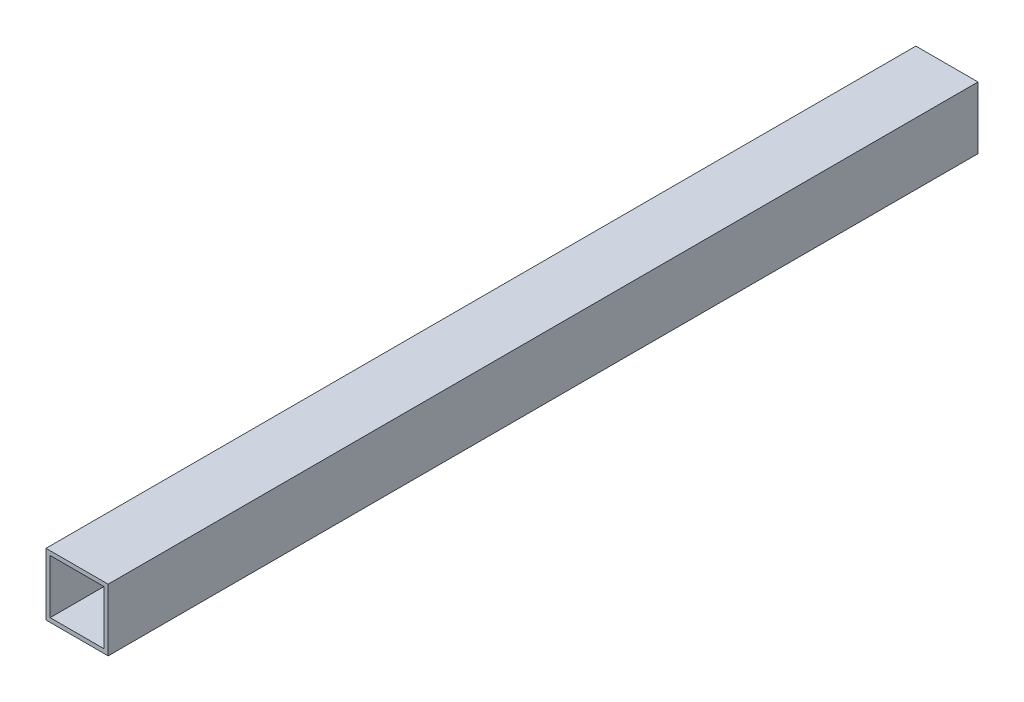
SolidWorks part; units mm, degrees
ref_plane "前视基准面" through (0, 0, 0) normal (0, 0, 1) x (1, 0, 0)
ref_plane "上视基准面" through (0, 0, 0) normal (0, 1, 0) x (1, 0, 0)
ref_plane "右视基准面" through (0, 0, 0) normal (1, 0, 0) x (0, 0, -1)
sketch "草图1" plane through (0, 0, 0) normal (0, 0, 1) x (1, 0, 0)
  line L0 (13, 13) -> (-13, 13)
  line L1 (15, -15) -> (-15, -15)
  line L2 (15, -15) -> (15, 15)
  line L3 (15, 15) -> (-15, 15)
  line L4 (-15, -15) -> (-15, 15)
  line L5 (15, -15) -> (-15, 15) construction
  line L6 (15, 15) -> (-15, -15) construction
  line L7 (-13, -13) -> (-13, 13)
  line L8 (13, -13) -> (-13, -13)
  line L9 (13, -13) -> (13, 13)
  point P0 (0, 0)
  dimension "D1" = 30
  dimension "D2" = 2
extrude "凸台-拉伸1" add sketch "草图1" along normal mid plane 420
sketch "草图2" plane through (0, 0, 210) normal (0, 0, 1) x (1, 0, 0)
  circle A1 centre (0, 0) radius 2.0463
